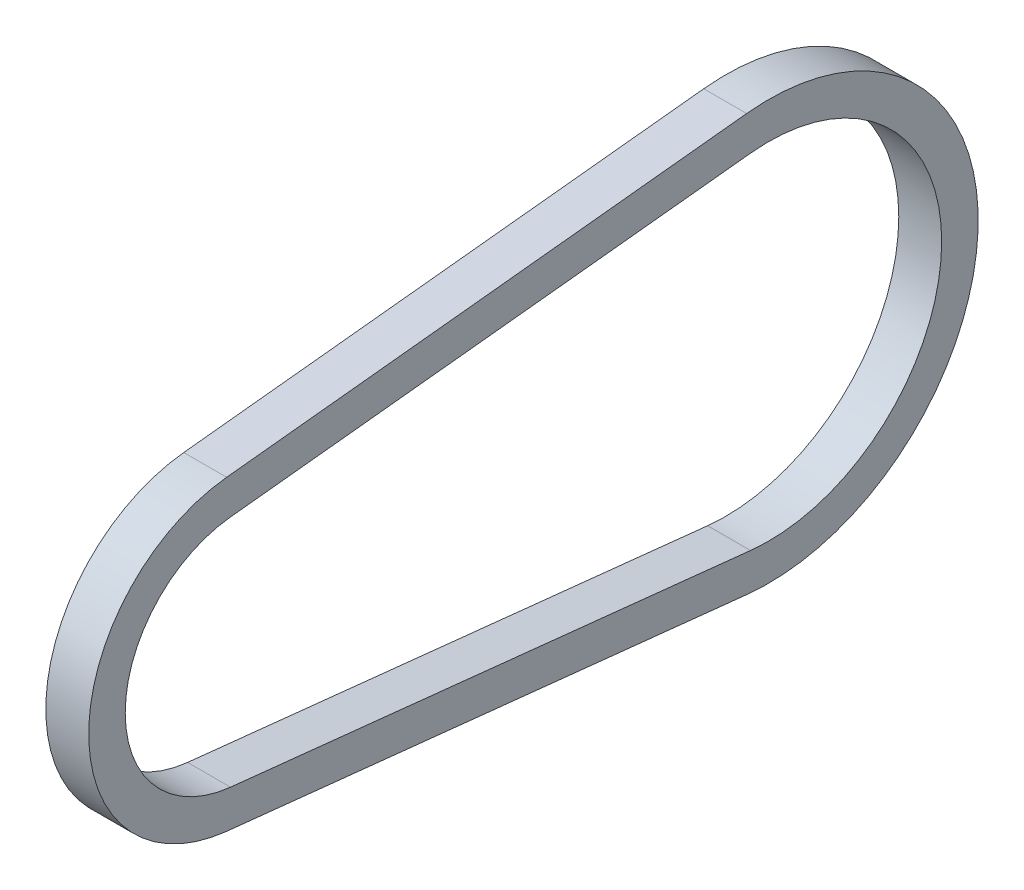
from build123d import *

# Parameters (mm, degrees)
EXTRUDE_1_DEPTH = 18.8


with BuildPart() as part:
    # 草图1 → 拉伸-薄壁1 (new body)
    with BuildSketch(Plane(origin=(0, 0, 0), x_dir=(0, 0, -1), z_dir=(1, 0, 0))):
        with BuildLine():
            Line((138.314113207, -107.167648268), (-89.533532193, -83.052342215))
            ThreePointArc((-89.533532193, -83.052342215), (-149.973777418, -15.877541233), (-89.533532193, 51.29725975))
            Line((-89.533532193, 51.29725975), (138.314113207, 75.412565802))
            ThreePointArc((138.314113207, 75.412565802), (239.776222582, -15.877541233), (138.314113207, -107.167648268))
        make_face()
        with BuildLine():
            Line((139.998140985, -91.256518501), (-87.849504415, -67.141212449))
            ThreePointArc((-87.849504415, -67.141212449), (-133.973777418, -15.877541233), (-87.849504415, 35.386129983))
            Line((-87.849504415, 35.386129983), (139.998140985, 59.501436035))
            ThreePointArc((139.998140985, 59.501436035), (223.776222582, -15.877541233), (139.998140985, -91.256518501))
        make_face(mode=Mode.SUBTRACT)
    extrude(amount=EXTRUDE_1_DEPTH)


solid = part.part
